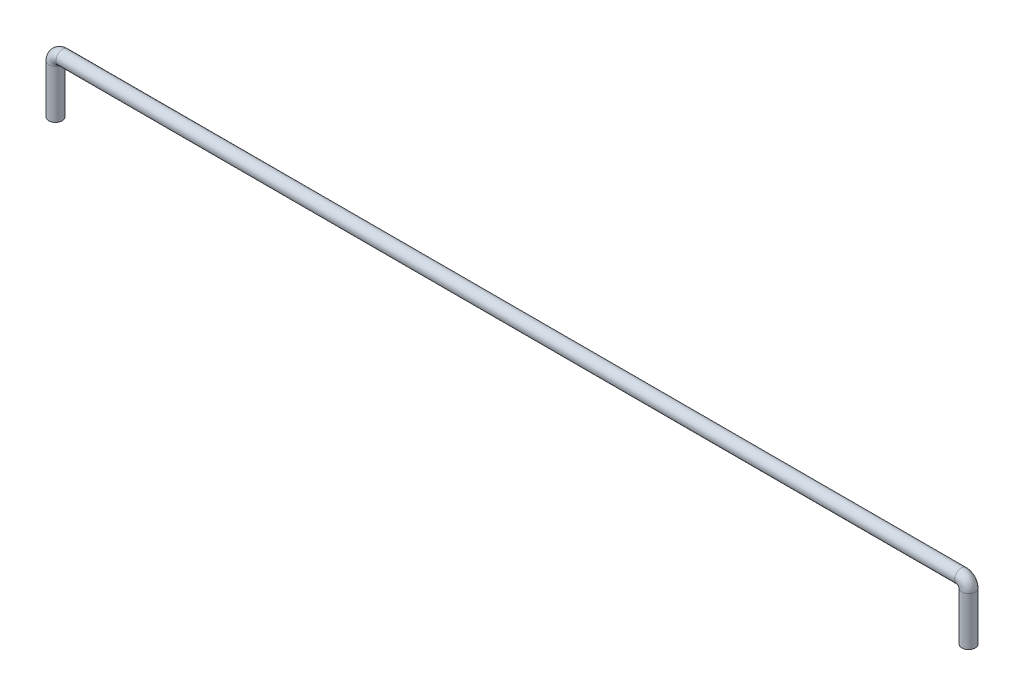
from build123d import *

# Parameters (mm, degrees)
SKETCH2_R = 6


with BuildPart() as part:
    # Sweep1: sweep along a path in Sketch1
    with BuildLine(Plane.XY) as sweep1_path:
        Line((-49.237651445, -16.859273066), (-49.237651445, 26.640726934))
        ThreePointArc((-49.237651445, 26.640726934), (-47.333845522, 31.236921012), (-42.737651445, 33.140726934))
        Line((-42.737651445, 33.140726934), (763.262348555, 33.140726934))
        ThreePointArc((763.262348555, 33.140726934), (767.858542633, 31.236921012), (769.762348555, 26.640726934))
        Line((769.762348555, 26.640726934), (769.762348555, -16.859273066))
    # Sketch2 → Sweep1 (sweep)
    with BuildSketch(Plane(origin=(-49.237651445, -16.859273066, 0), x_dir=(-1, 0, 0), z_dir=(0, 1, 0))):
        Circle(SKETCH2_R)
    sweep(path=sweep1_path.line)


solid = part.part
